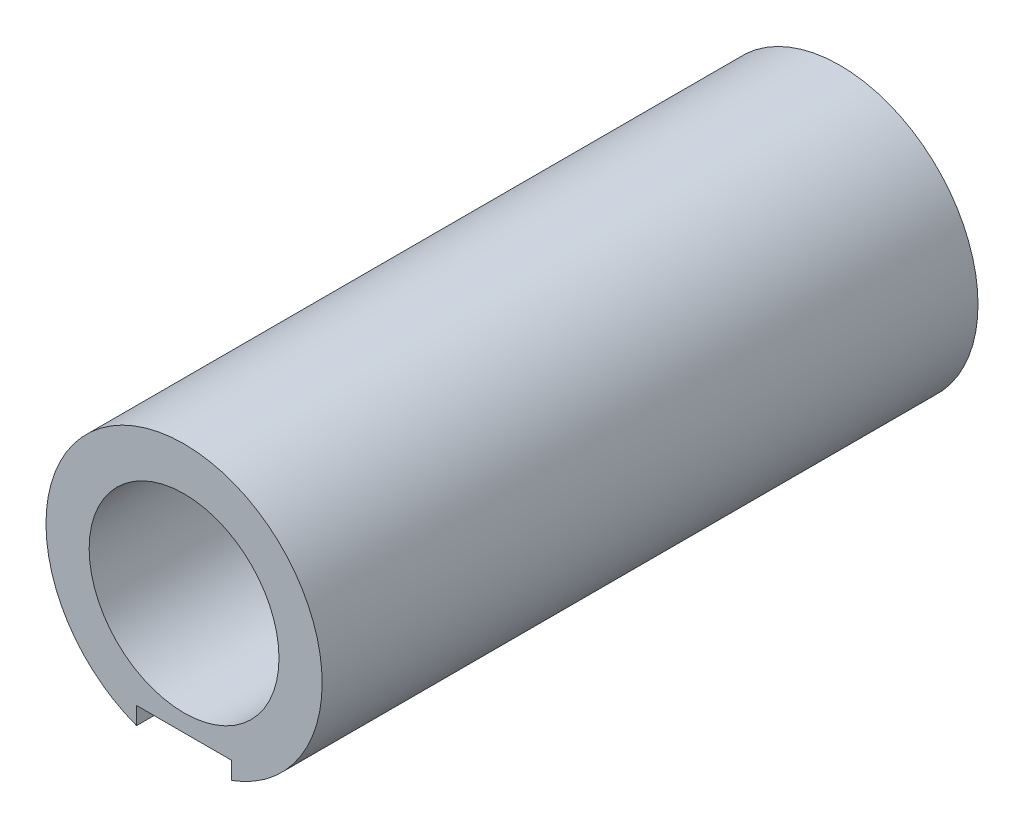
SolidWorks part; units mm, degrees
ref_plane "Front Plane" through (0, 0, 0) normal (0, 0, 1) x (1, 0, 0)
ref_plane "Top Plane" through (0, 0, 0) normal (0, 1, 0) x (1, 0, 0)
ref_plane "Right Plane" through (0, 0, 0) normal (1, 0, 0) x (0, 0, -1)
other "Configuration Table"
sketch "Sketch1" plane through (0, 0, 0) normal (0, 0, 1) x (1, 0, 0)
  circle A0 centre (-599.8842, -90) radius 80
extrude "Boss-Extrude1" add sketch "Sketch1" along normal blind 380
sketch "Sketch2" plane through (0, 0, 380) normal (0, 0, 1) x (1, 0, 0)
  line L1 (-572.3842, -185) -> (-627.3842, -185)
  line L2 (-572.3842, -185) -> (-572.3842, -155)
  line L3 (-572.3842, -155) -> (-627.3842, -155)
  line L4 (-627.3842, -185) -> (-627.3842, -155)
  line L5 (-572.3842, -185) -> (-627.3842, -155) construction
  line L6 (-572.3842, -155) -> (-627.3842, -185) construction
  circle A0 centre (-599.8842, -90) radius 80
  point P3 (-599.8842, -170)
  circle M3 centre (-599.8842, -90) radius 80
  dimension "D1" = 30
  dimension "D2" = 55
extrude "Cut-Extrude1" cut sketch "Sketch2" against normal blind 97 contours L4 L2 L3 M3
sketch "Sketch3" plane through (0, 0, 380) normal (0, 0, 1) x (1, 0, 0)
  circle A0 centre (-599.8842, -90) radius 55
  dimension "D1" = 110
extrude "Cut-Extrude2" cut sketch "Sketch3" against normal through all both and the other way through all
